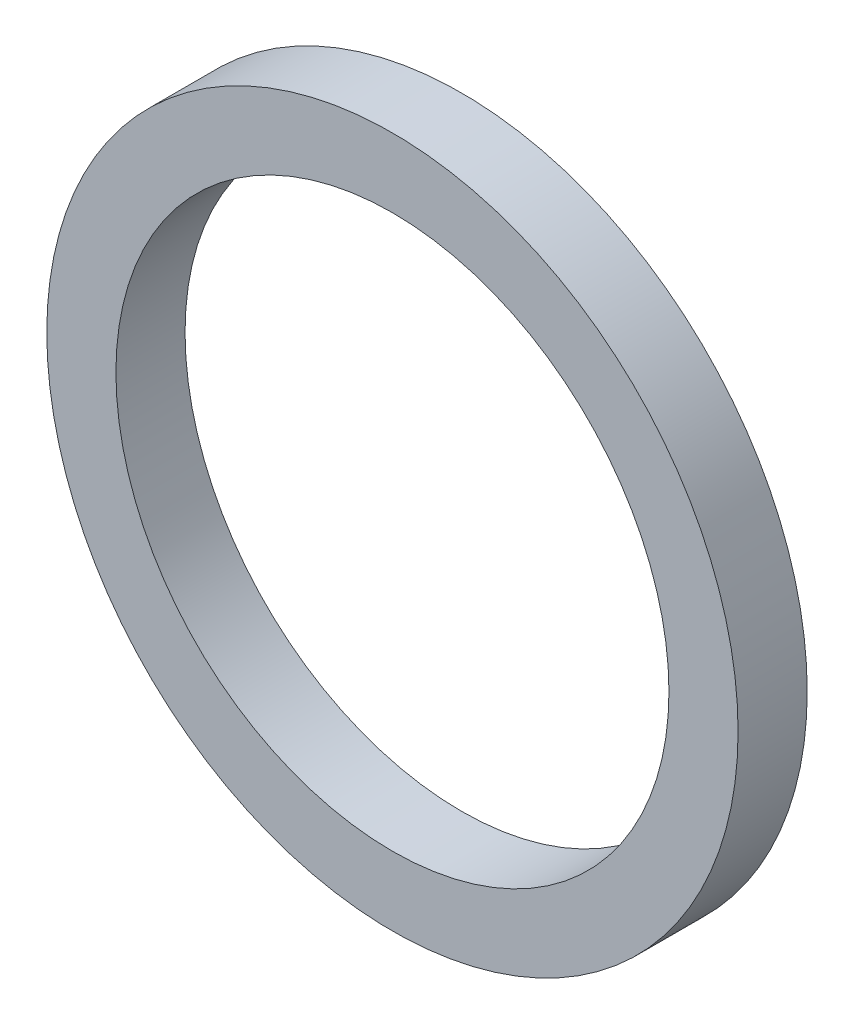
from build123d import *

# Parameters (mm, degrees)
SKETCH_1_R      = 25
SKETCH_1_R_2    = 20
EXTRUDE_1_DEPTH = 5


with BuildPart() as part:
    # 草图1 → 凸台-拉伸1 (new body)
    with BuildSketch(Plane.XY):
        Circle(SKETCH_1_R)
        Circle(SKETCH_1_R_2, mode=Mode.SUBTRACT)
    extrude(amount=EXTRUDE_1_DEPTH)


solid = part.part
